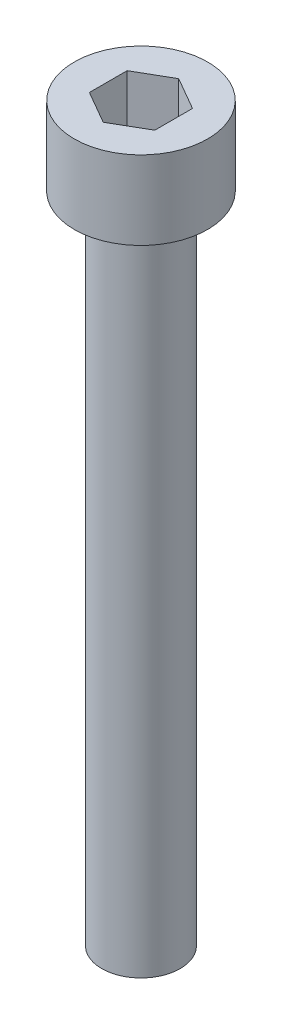
from build123d import *

# Parameters (mm, degrees)
CUT_EXTRUDE_1_DEPTH = 5


with BuildPart() as part:
    # Sketch 1 → Revolve 1 (revolve)
    with BuildSketch(Plane.XY, mode=Mode.PRIVATE) as revolve_1_sk:
        Polygon((0, 6), (-5.1, 6), (-5.1, 0), (-3, 0), (-3, -50), (0, -50), align=None)
    revolve(revolve_1_sk.sketch.rotate(Axis((0, 11.322033898, 0), (0, -1, 0)), 270), axis=Axis((0, 11.322033898, 0), (0, -1, 0)))

    # Sketch 2 → Cut-Extrude 1 (cut)
    with BuildSketch(Plane(origin=(0, 6, 0), x_dir=(1, 0, 0), z_dir=(0, 1, 0))):
        Polygon((0, 2.886751346), (-2.5, 1.443375673), (-2.5, -1.443375673), (0, -2.886751346), (2.5, -1.443375673), (2.5, 1.443375673), align=None)
    extrude(amount=-CUT_EXTRUDE_1_DEPTH, mode=Mode.SUBTRACT)


solid = part.part
